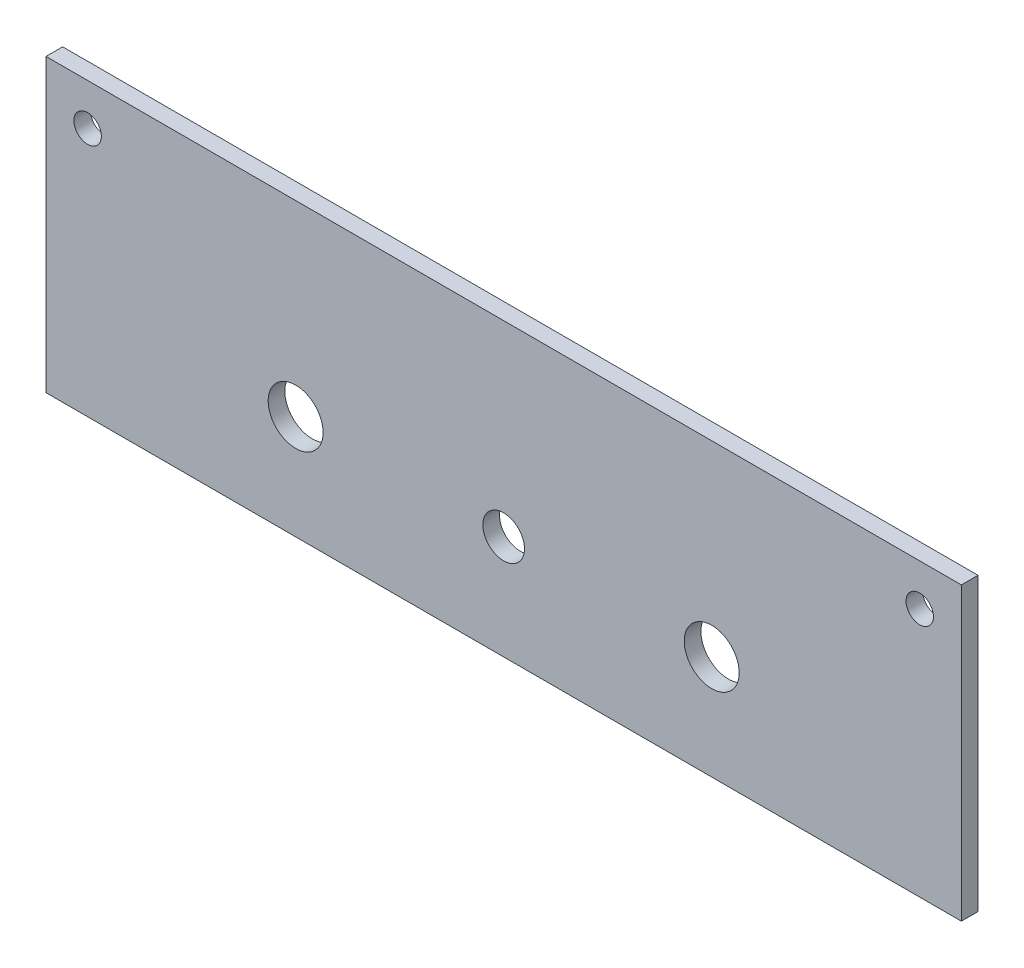
from build123d import *

# Parameters (mm, degrees)
SKETCH_1_W          = 110
SKETCH_1_H          = 25
SKETCH_1_R          = 3.3
EXTRUDE_1_DEPTH     = 1
SKETCH_2_R          = 2.5
CUT_EXTRUDE_1_DEPTH = 10
SKETCH_3_W          = 110
SKETCH_3_H          = 2
EXTRUDE_2_DEPTH     = 10
SKETCH_4_R          = 1.65
CUT_EXTRUDE_2_DEPTH = 10


with BuildPart() as part:
    # 草图1 → 凸台-拉伸1 (new, symmetric)
    with BuildSketch(Plane.XY):
        Rectangle(SKETCH_1_W, SKETCH_1_H)
        with Locations((-25, 0)):
            Circle(SKETCH_1_R, mode=Mode.SUBTRACT)
        with Locations((25, 0)):
            Circle(SKETCH_1_R, mode=Mode.SUBTRACT)
    extrude(amount=EXTRUDE_1_DEPTH, both=True)

    # 草图2 → 切除-拉伸1 (cut)
    with BuildSketch(Plane.XY.offset(1)):
        Circle(SKETCH_2_R)
    extrude(amount=-CUT_EXTRUDE_1_DEPTH, mode=Mode.SUBTRACT)

    # 草图3 → 凸台-拉伸2 (add)
    with BuildSketch(Plane(origin=(0, 12.5, 0), x_dir=(1, 0, 0), z_dir=(0, 1, 0))):
        Rectangle(SKETCH_3_W, SKETCH_3_H)
    extrude(amount=EXTRUDE_2_DEPTH)

    # 草图4 → 切除-拉伸2 (cut)
    with BuildSketch(Plane(origin=(0, 0, -1), x_dir=(-1, 0, 0), z_dir=(0, 0, -1))):
        with Locations((-50, 17.5)):
            Circle(SKETCH_4_R)
        with Locations((50, 17.5)):
            Circle(SKETCH_4_R)
    extrude(amount=-CUT_EXTRUDE_2_DEPTH, mode=Mode.SUBTRACT)


solid = part.part
